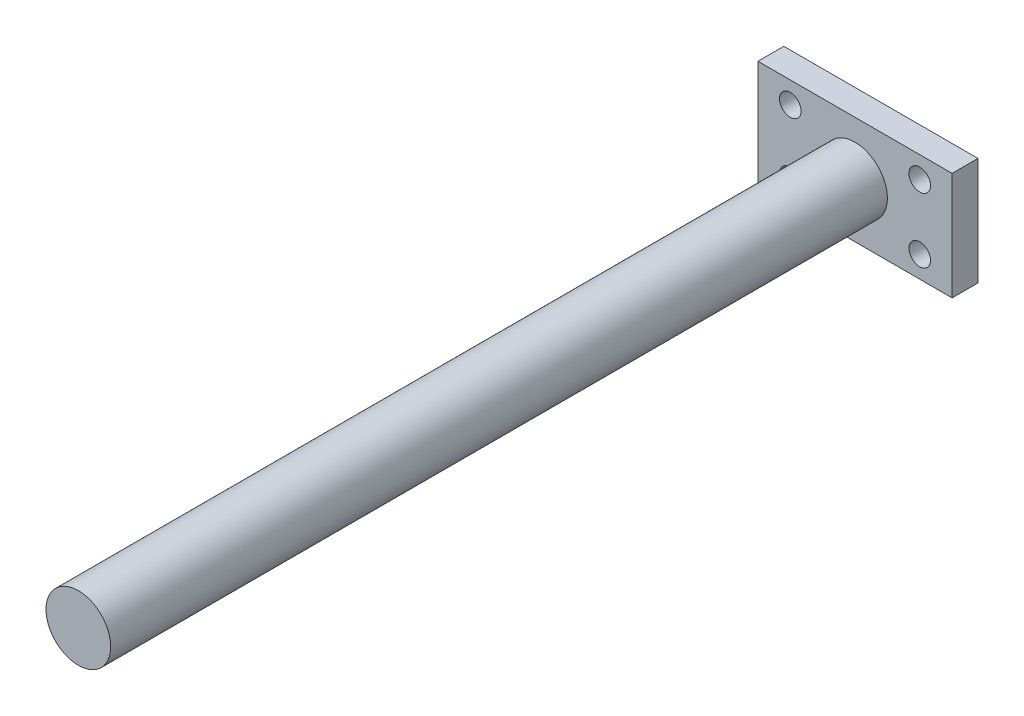
SolidWorks part; units mm, degrees
ref_plane "Front Plane" through (0, 0, 0) normal (0, 0, 1) x (1, 0, 0)
ref_plane "Top Plane" through (0, 0, 0) normal (0, 1, 0) x (1, 0, 0)
ref_plane "Right Plane" through (0, 0, 0) normal (1, 0, 0) x (0, 0, -1)
other "Configuration Table"
sketch "Sketch1" plane through (0, 0, 0) normal (0, 0, 1) x (1, 0, 0)
  line L1 (-45, 25) -> (45, 25)
  line L2 (-45, 25) -> (-45, -25)
  line L3 (-45, -25) -> (45, -25)
  line L4 (45, 25) -> (45, -25)
  line L5 (-45, 25) -> (45, -25) construction
  line L6 (-45, -25) -> (45, 25) construction
  line L7 (-30, 15) -> (30, 15) construction
  line L8 (-30, 15) -> (-30, -15) construction
  line L9 (-30, -15) -> (30, -15) construction
  line L10 (30, 15) -> (30, -15) construction
  line L11 (-30, 15) -> (30, -15) construction
  line L12 (-30, -15) -> (30, 15) construction
  circle A0 centre (-30, 15) radius 5
  circle A1 centre (-30, -15) radius 5
  circle A2 centre (30, -15) radius 5
  circle A3 centre (30, 15) radius 5
  point P0 (0, 0)
  point P6 (0, 0)
  dimension "D5" = 10
  dimension "D1" = 90
  dimension "D2" = 50
  dimension "D3" = 10
  dimension "D4" = 15
extrude "Boss-Extrude1" add sketch "Sketch1" along normal blind 12
sketch "Sketch2" plane through (0, 0, 12) normal (0, 0, 1) x (1, 0, 0)
  circle A0 centre (0, 0) radius 15
  dimension "D1" = 30
extrude "Boss-Extrude2" add sketch "Sketch2" along normal blind 360
